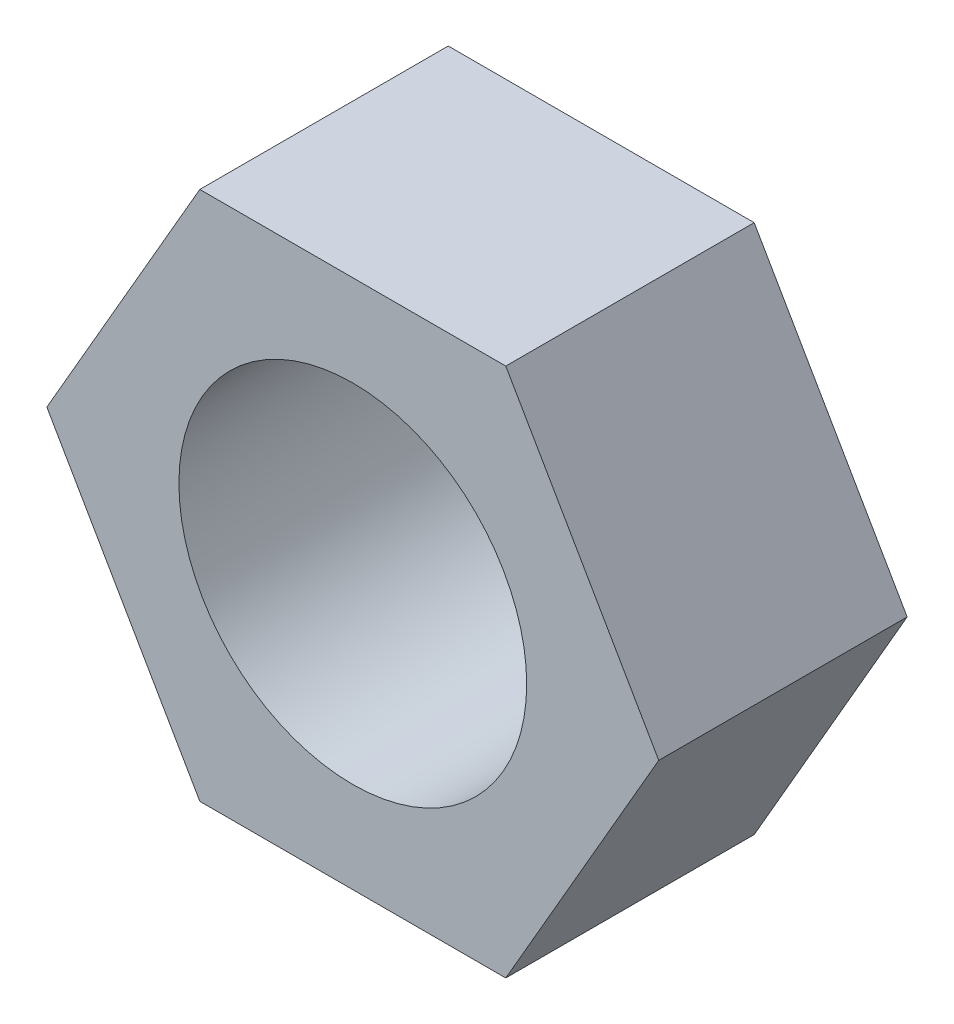
SolidWorks part; units mm, degrees
ref_plane "Front Plane" through (0, 0, 0) normal (0, 0, 1) x (1, 0, 0)
ref_plane "Top Plane" through (0, 0, 0) normal (0, 1, 0) x (1, 0, 0)
ref_plane "Right Plane" through (0, 0, 0) normal (1, 0, 0) x (0, 0, -1)
sketch "Sketch1" plane through (0, 0, 0) normal (0, 0, 1) x (1, 0, 0)
  line L1 (18.4752, 0) -> (9.2376, 16)
  line L2 (9.2376, 16) -> (-9.2376, 16)
  line L3 (-9.2376, 16) -> (-18.4752, 0)
  line L4 (-18.4752, 0) -> (-9.2376, -16)
  line L5 (-9.2376, -16) -> (9.2376, -16)
  line L6 (9.2376, -16) -> (18.4752, 0)
  circle A0 centre (0, 0) radius 16 construction
  dimension "D1" = 32
extrude "Boss-Extrude1" add sketch "Sketch1" along normal blind 15
hole_wizard "M24 Tapped Hole1" positions "Sketch3" profile "Sketch2" tap size "M24" standard "GB"
sketch "Sketch3" plane through (0, 0, 15) normal (0, 0, 1) x (1, 0, 0)
  point P0 (0, 0)
sketch "Sketch2" plane through (0, 0, 15) normal (1, 0, 0) x (0, -1, 0)
  line L0 (0, 0) -> (0, 63.309)
  line L1 (0, 63.309) -> (10.5, 57)
  line L2 (10.5, 57) -> (10.5, 0)
  line L5 (10.5, 0) -> (0, 0)
  line L10 (0, 63.309) -> (-10.5, 57) construction
  line L11 (0, -6.35) -> (0, 107.95) construction
  dimension "螺纹孔钻头直径" = 21
  dimension "螺纹孔钻头深度" = 57
  dimension "导头角度" = 118
cosmetic thread "Cosmetic Thread1"
